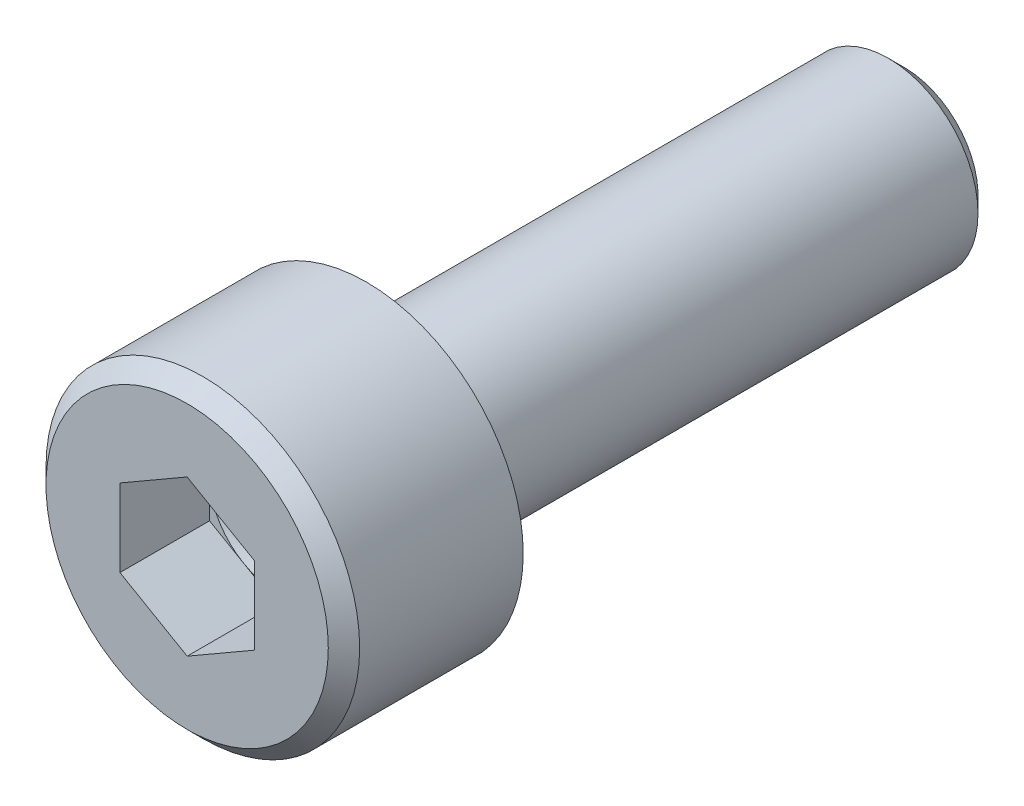
from build123d import *

# Parameters (mm, degrees)
SKETCH_1_W          = 3.5
SKETCH_1_H          = 4
SKETCH_2_R          = 2
EXTRUDE_1_DEPTH     = 12
CUT_EXTRUDE_1_DEPTH = 2
CHAMFER_1_SIZE      = 0.35


with BuildPart() as part:
    # 草图1 → 旋转1 (revolve)
    with BuildSketch(Plane(origin=(0, 0, 0), x_dir=(1, 0, 0), z_dir=(0, 1, 0))):
        with Locations((1.75, -2)):
            Rectangle(SKETCH_1_W, SKETCH_1_H)
    revolve(axis=Axis((0, 0, 0), (0, 0, 1)))

    # 草图2 → 凸台-拉伸1 (add)
    with BuildSketch(Plane(origin=(0, 0, 0), x_dir=(-1, 0, 0), z_dir=(0, 0, -1))):
        Circle(SKETCH_2_R)
    extrude(amount=EXTRUDE_1_DEPTH)

    # 草图3 → 切除-拉伸1 (cut)
    with BuildSketch(Plane.XY.offset(4)):
        Polygon((1.5, -0.866025404), (1.5, 0.866025404), (0, 1.732050808), (-1.5, 0.866025404), (-1.5, -0.866025404), (0, -1.732050808), align=None)
    extrude(amount=-CUT_EXTRUDE_1_DEPTH, mode=Mode.SUBTRACT)

    # 草图4 → 切除-旋转1 (revolve, cut)
    with BuildSketch(Plane.XZ, mode=Mode.PRIVATE) as cut_revolve_1_sk:
        Polygon((1.5, 2), (0, 2), (0, 1.133974596), align=None)
    revolve(cut_revolve_1_sk.sketch.rotate(Axis((0, 0, 2), (0, 0, -1)), 90), axis=Axis((0, 0, 2), (0, 0, -1)), mode=Mode.SUBTRACT)

    # 倒角1
    chamfer_1_edges = [part.edges().sort_by_distance(p)[0] for p in [
        (-3.5, 0, 4),
        (2, 0, -12),
    ]]
    chamfer(chamfer_1_edges, length=CHAMFER_1_SIZE)


solid = part.part
